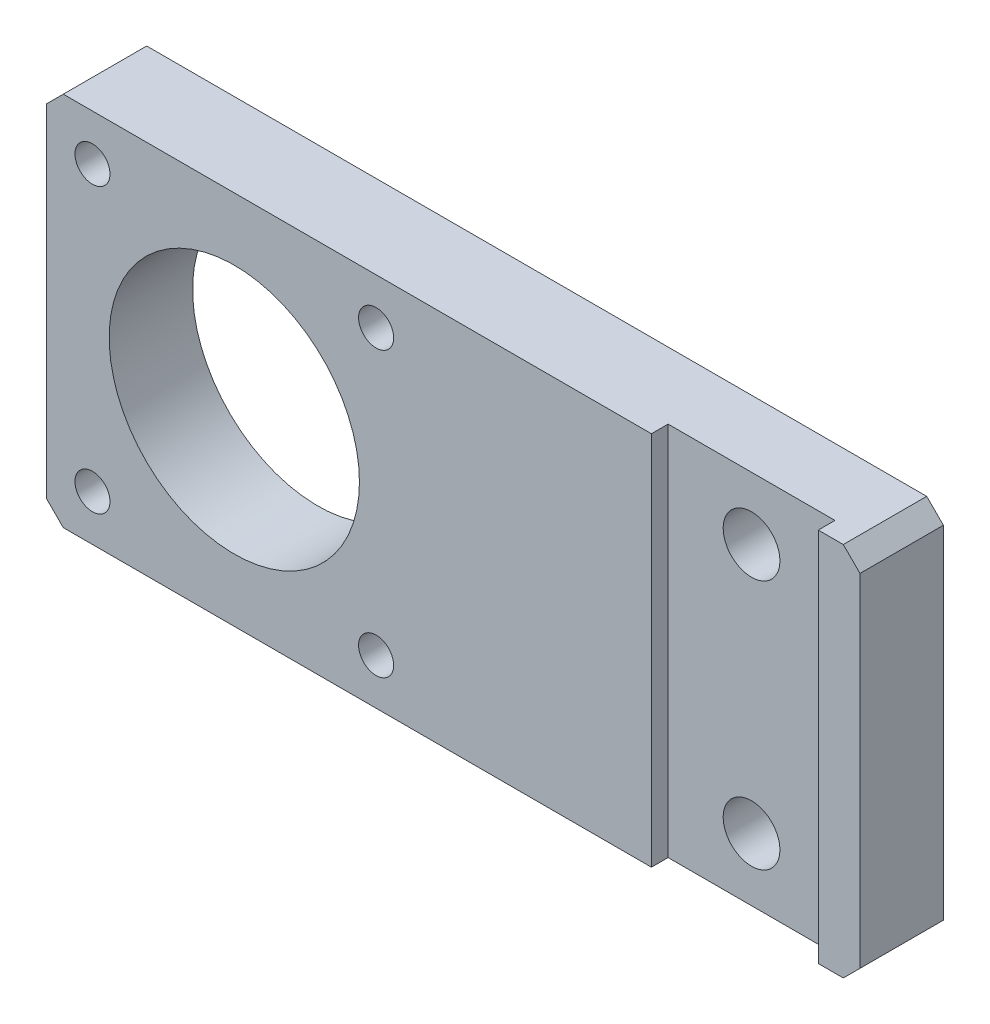
SolidWorks part; units mm, degrees
ref_plane "Front Plane" through (0, 0, 0) normal (0, 0, 1) x (1, 0, 0)
ref_plane "Top Plane" through (0, 0, 0) normal (0, 1, 0) x (1, 0, 0)
ref_plane "Right Plane" through (0, 0, 0) normal (1, 0, 0) x (0, 0, -1)
sketch "Sketch1" plane through (0, 0, 0) normal (0, 0, 1) x (1, 0, 0)
  line L1 (0, 0) -> (97.5, 0)
  line L2 (0, 0) -> (0, 45)
  line L3 (0, 45) -> (97.5, 45)
  line L4 (97.5, 0) -> (97.5, 45)
  circle A0 centre (22.5, 22.5) radius 15
  circle A1 centre (82.5, 37.5) radius 3.4
  circle A2 centre (82.5, 7.5) radius 3.4
  dimension "D3" = 30
  dimension "D6" = 6.8
  dimension "D1" = 45
  dimension "D2" = 97.5
  dimension "D4" = 22.5
  dimension "D5" = 22.5
  dimension "D7" = 30
  dimension "D8" = 7.5
  dimension "D9" = 15
extrude "Boss-Extrude1" add sketch "Sketch1" along normal blind 10
sketch "Sketch2" plane through (0, 45, 0) normal (0, 1, 0) x (1, 0, 0)
  line L0 (97.5, -10) -> (0, -10) construction
  line L1 (72.5, -10) -> (92.5, -10)
  line L2 (72.5, -10) -> (72.5, -8)
  line L3 (72.5, -8) -> (92.5, -8)
  line L4 (92.5, -10) -> (92.5, -8)
  line L5 (97.5, -10) -> (97.5, 0) construction
  dimension "D1" = 20
  dimension "D2" = 5
  dimension "D3" = 2
extrude "Cut-Extrude1" cut sketch "Sketch2" against normal up to next
hole_wizard "M5 Tapped Hole1" positions "Sketch4" profile "Sketch3" tap size "M5" standard "GB"
sketch "Sketch4" plane through (0, 0, 0) normal (0, 0, -1) x (-1, 0, 0)
  circle A0 centre (-22.5, 22.5) radius 15 construction
  point P0 (-39.5, 5.5)
  point P1 (-5.5, 5.5)
  point P3 (-5.5, 39.5)
  point P5 (-39.5, 39.5)
  dimension "D3" = 17
  dimension "D1" = 34
  dimension "D2" = 34
  dimension "D4" = 17
sketch "Sketch3" plane through (39.5, 5.5, 0) normal (1, 0, 0) x (0, 1, 0)
  line L0 (0, 0) -> (0, 13.6618)
  line L1 (0, 13.6618) -> (2.1, 12.4)
  line L2 (2.1, 12.4) -> (2.1, 0)
  line L5 (2.1, 0) -> (0, 0)
  line L10 (0, 13.6618) -> (-2.1, 12.4) construction
  line L11 (0, -6.35) -> (0, 107.95) construction
  dimension "螺纹孔钻头直径" = 4.2
  dimension "螺纹孔钻头深度" = 12.4
  dimension "导头角度" = 118
cosmetic thread "Cosmetic Thread1" parameters "D1"=10, "D2"=5
cosmetic thread "Cosmetic Thread2" parameters "D1"=10, "D2"=5
cosmetic thread "Cosmetic Thread3" parameters "D1"=10, "D2"=5
cosmetic thread "Cosmetic Thread4" parameters "D1"=10, "D2"=5
chamfer "Chamfer1" distance 2 angle 45 4 edges at (97.5, 0, 5) (97.5, 45, 5) (0, 0, 5) (0, 45, 5)
